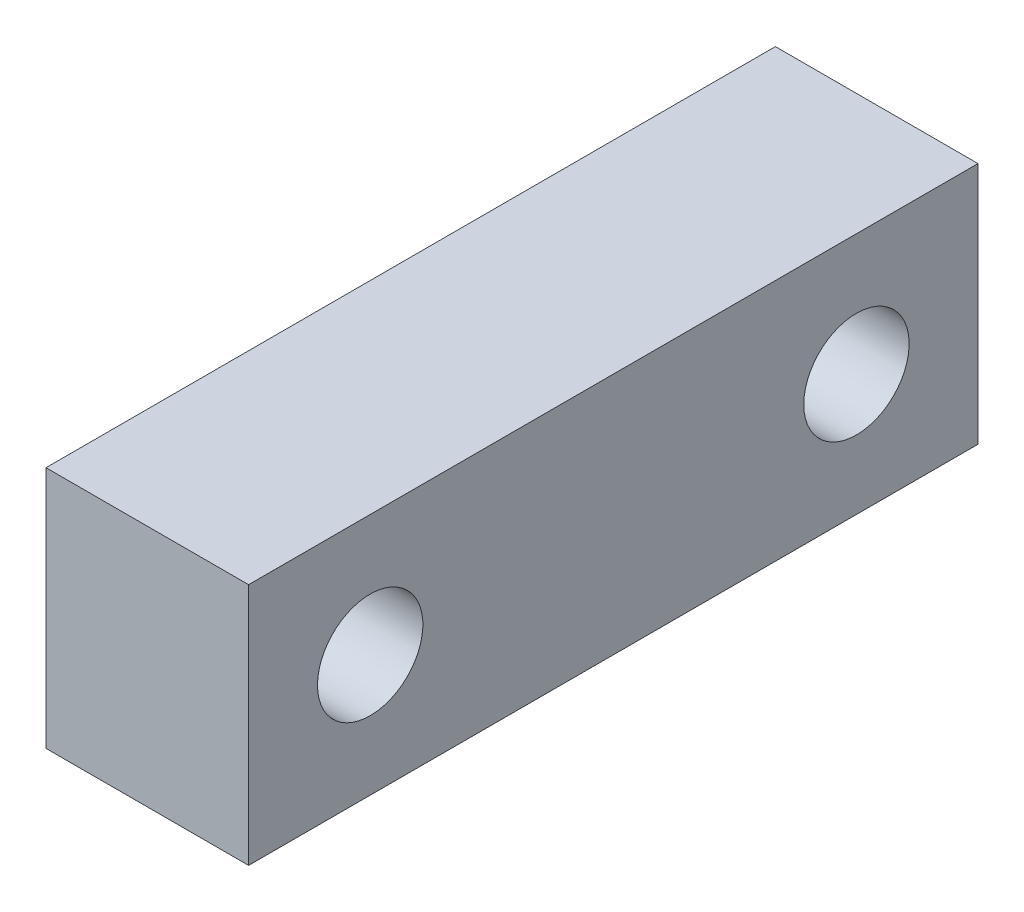
SolidWorks part; units mm, degrees
ref_plane "Front Plane" through (0, 0, 0) normal (0, 0, 1) x (1, 0, 0)
ref_plane "Top Plane" through (0, 0, 0) normal (0, 1, 0) x (1, 0, 0)
ref_plane "Right Plane" through (0, 0, 0) normal (1, 0, 0) x (0, 0, -1)
sketch "Sketch1" plane through (0, 0, 0) normal (0, 1, 0) x (1, 0, 0)
  line L1 (-2.5, 9) -> (2.5, 9)
  line L2 (-2.5, 9) -> (-2.5, -9)
  line L3 (-2.5, -9) -> (2.5, -9)
  line L4 (2.5, 9) -> (2.5, -9)
  line L5 (-2.5, 9) -> (2.5, -9) construction
  line L6 (-2.5, -9) -> (2.5, 9) construction
  point P0 (0, 0)
  dimension "D1" = 5
  dimension "D2" = 18
extrude "Boss-Extrude1" add sketch "Sketch1" along normal blind 6
sketch "Sketch2" plane through (-2.5, 0, 0) normal (-1, 0, 0) x (0, 0, 1)
  line L0 (0, 0) -> (0, 50000) construction
  line L1 (-9, 3) -> (49991, 3) construction
  line L2 (-9, 6) -> (-9, 0) construction
  line L3 (-9, 6) -> (9, 6) construction
  line L4 (-9, 0) -> (9, 0) construction
  circle A0 centre (6, 3) radius 1.3
  circle A1 centre (-6, 3) radius 1.3
  point P7 (-9, 3)
  dimension "D1" = 2.6
  dimension "D2" = 12
extrude "Cut-Extrude1" cut sketch "Sketch2" against normal blind 10
sketch "Sketch3" plane through (-2.5, 0, 0) normal (-1, 0, 0) x (0, 0, 1)
  circle A0 centre (-6, 3) radius 2.3
  circle A1 centre (6, 3) radius 2.3
  dimension "D1" = 4.6
extrude "Cut-Extrude2" cut sketch "Sketch3" against normal blind 3
